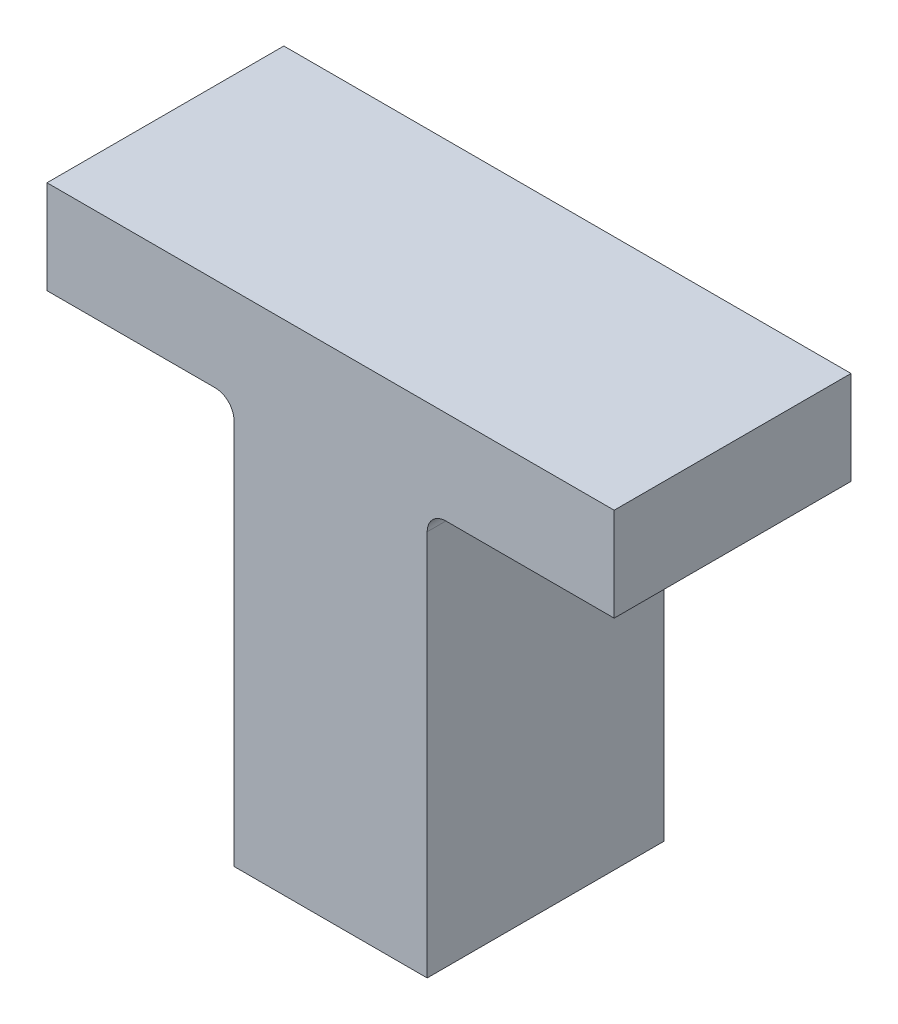
SolidWorks part; units mm, degrees
ref_plane "前视基准面" through (0, 0, 0) normal (0, 0, 1) x (1, 0, 0)
ref_plane "上视基准面" through (0, 0, 0) normal (0, 1, 0) x (1, 0, 0)
ref_plane "右视基准面" through (0, 0, 0) normal (1, 0, 0) x (0, 0, -1)
sketch "草图1" plane through (0, 0, 0) normal (0, 0, 1) x (1, 0, 0)
  line L1 (-45.5, -40) -> (45.5, -40)
  line L2 (-45.5, -40) -> (-45.5, 40)
  line L3 (-45.5, 40) -> (45.5, 40)
  line L4 (45.5, -40) -> (45.5, 40)
  line L5 (-45.5, -40) -> (45.5, 40) construction
  line L6 (-45.5, 40) -> (45.5, -40) construction
  point P0 (0, 0)
  dimension "D1" = 80
  dimension "D2" = 91
extrude "凸台-拉伸1" add sketch "草图1" along normal mid plane 38
sketch "草图2" plane through (0, 0, 19) normal (0, 0, 1) x (1, 0, 0)
  line L0 (45.5, 40) -> (-45.5, 40) construction
  line L1 (-45.5, -40) -> (-15.5, -40)
  line L2 (-45.5, -40) -> (-45.5, 25)
  line L3 (-45.5, 25) -> (-15.5, 25)
  line L4 (-15.5, -40) -> (-15.5, 25)
  line L5 (45.5, -40) -> (15.5, -40)
  line L6 (45.5, -40) -> (45.5, 25)
  line L7 (45.5, 25) -> (15.5, 25)
  line L8 (15.5, -40) -> (15.5, 25)
  dimension "D1" = 30
  dimension "D2" = 15
extrude "切除-拉伸1" cut sketch "草图2" against normal up to next
fillet "圆角1" radius 3 2 edges at (15.5, 25, 0) (-15.5, 25, 0)
